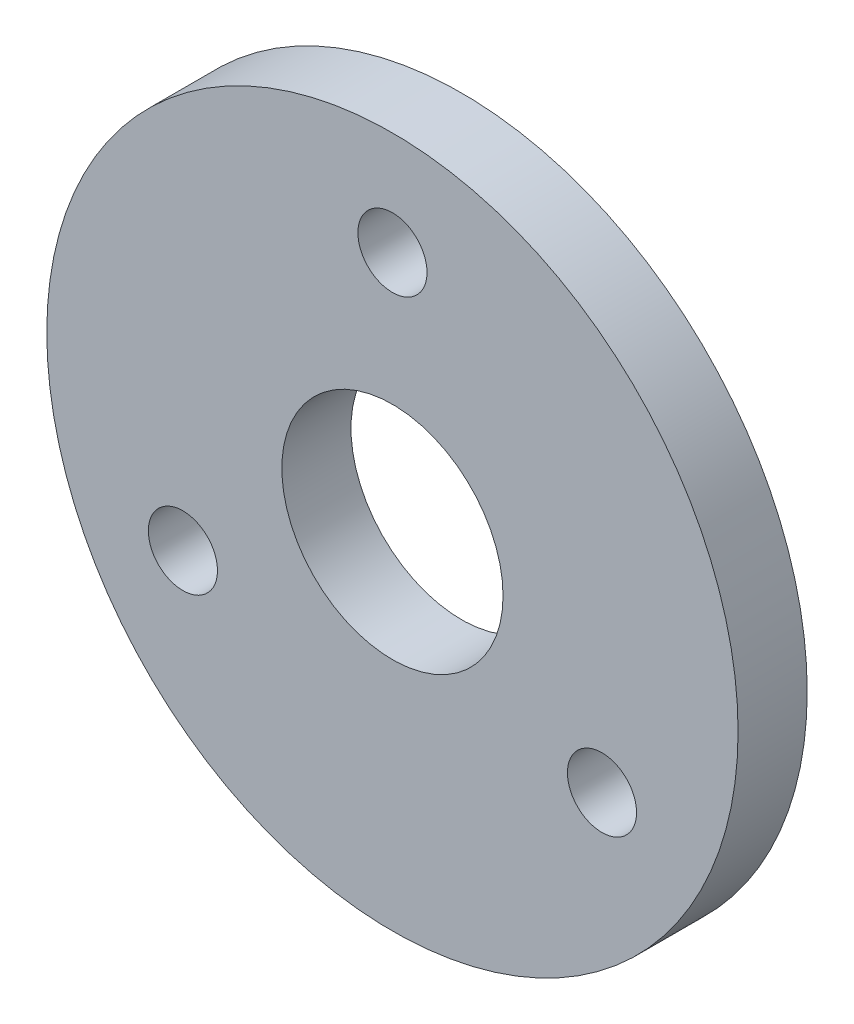
SolidWorks part; units mm, degrees
ref_plane "Front Plane" through (0, 0, 0) normal (0, 0, 1) x (1, 0, 0)
ref_plane "Top Plane" through (0, 0, 0) normal (0, 1, 0) x (1, 0, 0)
ref_plane "Right Plane" through (0, 0, 0) normal (1, 0, 0) x (0, 0, -1)
other "Configuration Table"
sketch "Sketch1" plane through (0, 0, 0) normal (0, 0, 1) x (1, 0, 0)
  circle A0 centre (0, 0) radius 50
  dimension "D1" = 100
extrude "Boss-Extrude1" add sketch "Sketch1" along normal blind 10
sketch "Sketch2" plane through (0, 0, 10) normal (0, 0, 1) x (1, 0, 0)
  circle A1 centre (0, 35) radius 5
  dimension "D2" = 10
extrude "Cut-Extrude1" cut sketch "Sketch2" against normal blind 10
pattern_circular "CirPattern1" count 3 over 360 about axis through (0, 0, 0) along (0, 0, 1) of "Cut-Extrude1"
sketch "Sketch3" plane through (0, 0, 10) normal (0, 0, 1) x (1, 0, 0)
  circle A0 centre (0, 0) radius 16
  dimension "D1" = 32
extrude "Cut-Extrude2" cut sketch "Sketch3" against normal blind 10
